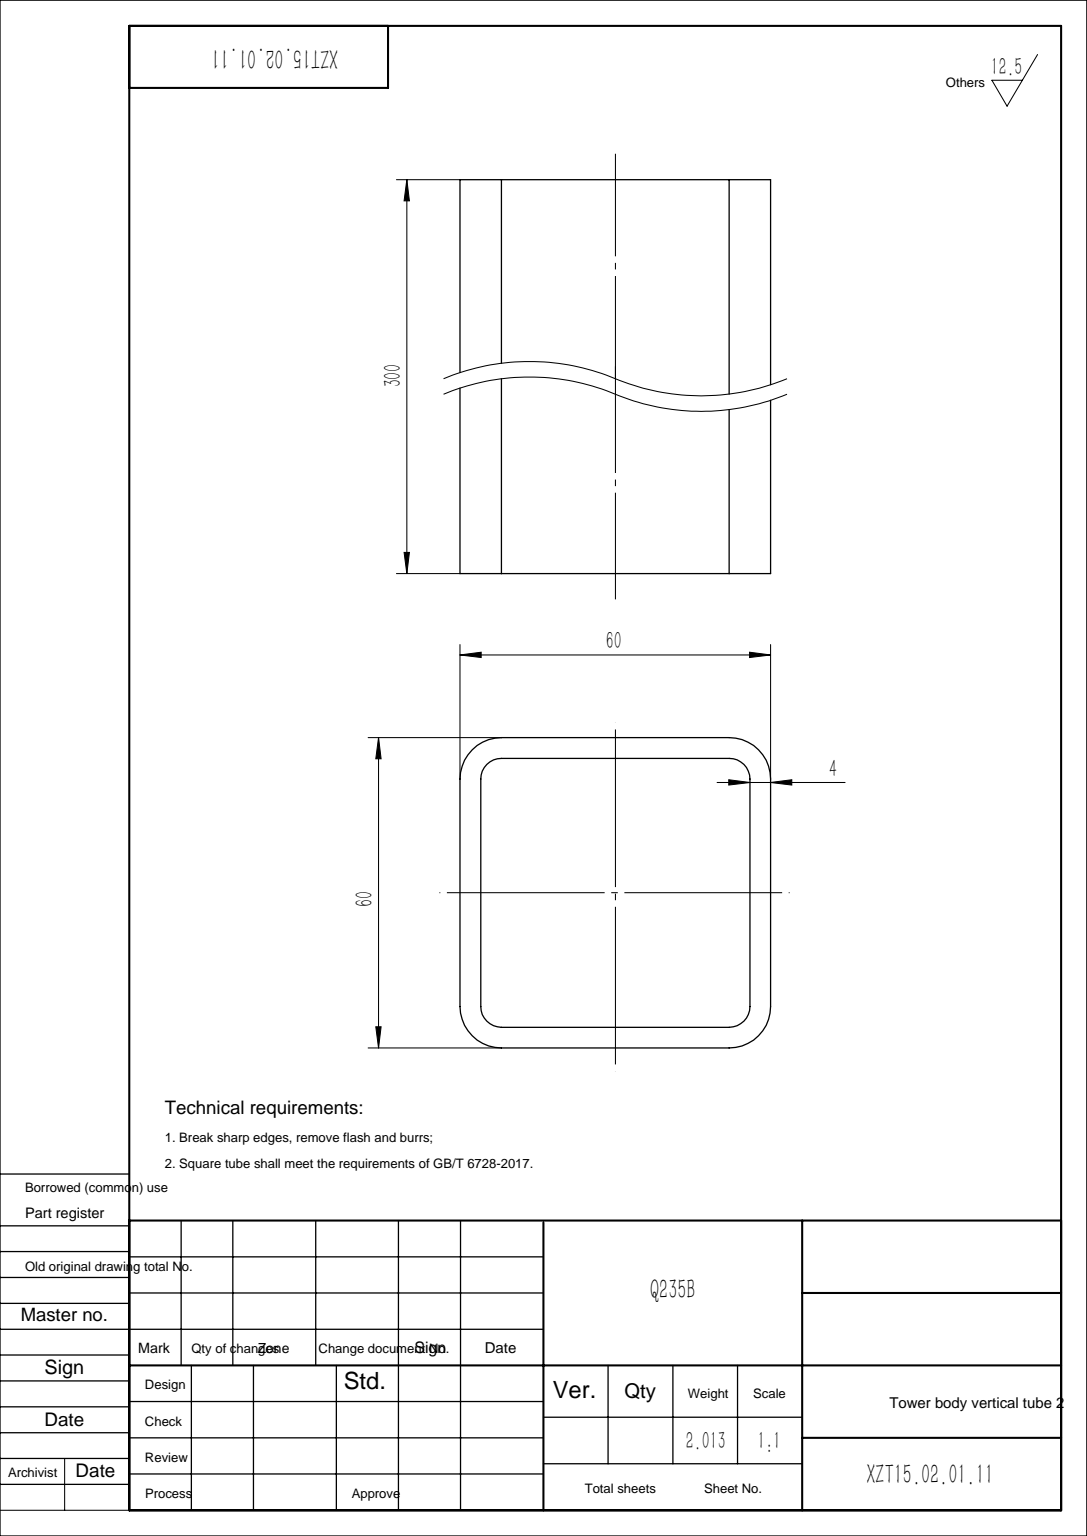
from build123d import *

# Parameters (mm, degrees)
GB_T_6728_2002_SQUARE_HOLLOW_SECTION_60_DEPTH = 300


with BuildPart() as part:
    # Sketch1 → GB/T 6728-2002 square hollow section 60×60×4(1) (new body)
    with BuildSketch(Plane(origin=(0, 0, 0), x_dir=(-1, 0, 0), z_dir=(0, 1, 0))):
        with BuildLine():
            Line((-22, -30), (22, -30))
            ThreePointArc((22, -30), (27.656854249, -27.656854249), (30, -22))
            Line((30, -22), (30, 22))
            ThreePointArc((30, 22), (27.656854249, 27.656854249), (22, 30))
            Line((22, 30), (-22, 30))
            ThreePointArc((-22, 30), (-27.656854249, 27.656854249), (-30, 22))
            Line((-30, 22), (-30, -22))
            ThreePointArc((-30, -22), (-27.656854249, -27.656854249), (-22, -30))
        make_face()
        with BuildLine():
            Line((-22, -26), (22, -26))
            ThreePointArc((22, -26), (24.828427125, -24.828427125), (26, -22))
            Line((26, -22), (26, 22))
            ThreePointArc((26, 22), (24.828427125, 24.828427125), (22, 26))
            Line((22, 26), (-22, 26))
            ThreePointArc((-22, 26), (-24.828427125, 24.828427125), (-26, 22))
            Line((-26, 22), (-26, -22))
            ThreePointArc((-26, -22), (-24.828427125, -24.828427125), (-22, -26))
        make_face(mode=Mode.SUBTRACT)
    extrude(amount=GB_T_6728_2002_SQUARE_HOLLOW_SECTION_60_DEPTH)


solid = part.part
